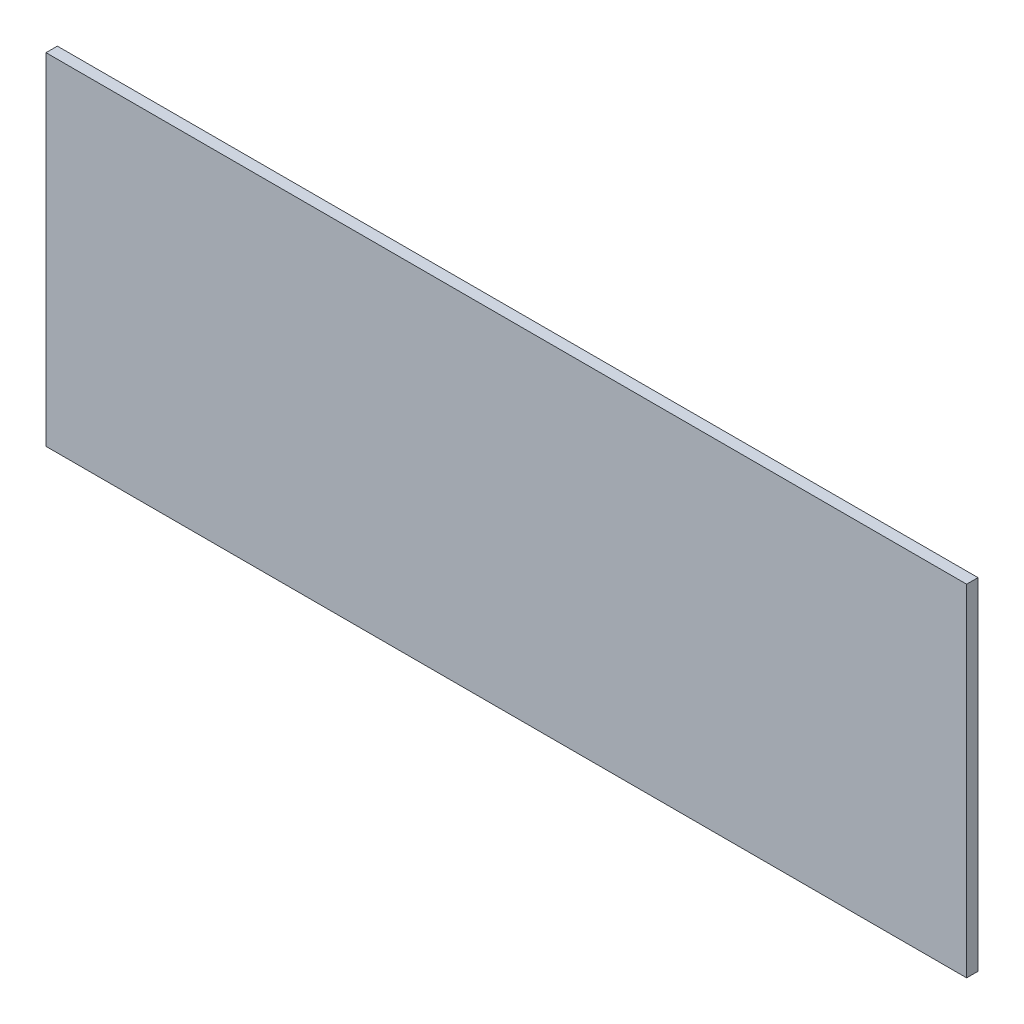
from build123d import *

# Parameters (mm, degrees)
SKETCH_1_W      = 405
SKETCH_1_H      = 150
EXTRUDE_1_DEPTH = 5


with BuildPart() as part:
    # 草图1 → 凸台-拉伸1 (new body)
    with BuildSketch(Plane.XY):
        Rectangle(SKETCH_1_W, SKETCH_1_H)
    extrude(amount=EXTRUDE_1_DEPTH)


solid = part.part
